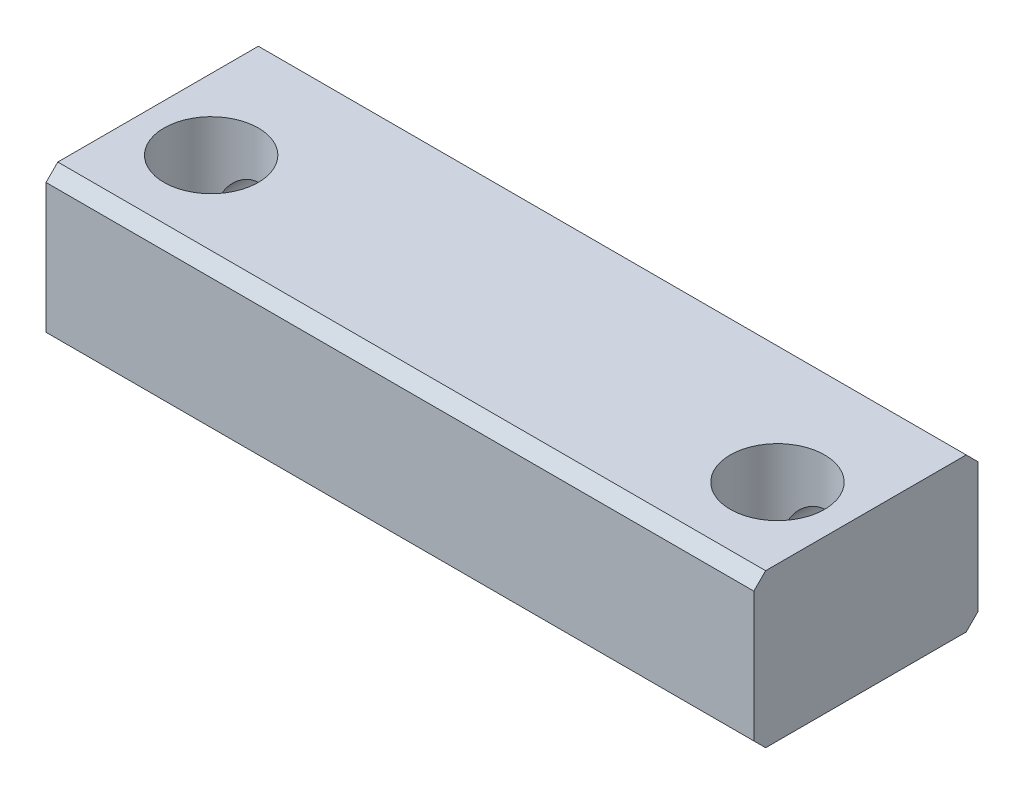
SolidWorks part; units mm, degrees
ref_plane "Front Plane" through (0, 0, 0) normal (0, 0, 1) x (1, 0, 0)
ref_plane "Top Plane" through (0, 0, 0) normal (0, 1, 0) x (1, 0, 0)
ref_plane "Right Plane" through (0, 0, 0) normal (1, 0, 0) x (0, 0, -1)
sketch "Sketch1" plane through (0, 0, 0) normal (0, 0, 1) x (1, 0, 0)
  line L1 (15, -3.25) -> (-15, -3.25)
  line L2 (15, -3.25) -> (15, 3.25)
  line L3 (15, 3.25) -> (-15, 3.25)
  line L4 (-15, -3.25) -> (-15, 3.25)
  line L5 (15, -3.25) -> (-15, 3.25) construction
  line L6 (15, 3.25) -> (-15, -3.25) construction
  point P0 (0, 0)
  dimension "D1" = 30
  dimension "D2" = 6.5
extrude "Boss-Extrude1" add sketch "Sketch1" along normal blind 9.5
sketch "Sketch2" plane through (0, 3.25, 0) normal (0, 1, 0) x (1, 0, 0)
  line L0 (15, 0) -> (-15, 0) construction
  line L1 (0, 0) -> (0, -9.5) construction
  line L2 (15, -9.5) -> (-15, -9.5) construction
  circle A0 centre (-12, -5.5) radius 2
  circle A1 centre (12, -5.5) radius 2
  dimension "D1" = 4
  dimension "D2" = 24
  dimension "D3" = 5.5
extrude "Cut-Extrude1" cut sketch "Sketch2" against normal through all
hole_wizard "M3 Tapped Hole1" positions "Sketch4" profile "Sketch3" tap size "M3" standard "GB"
sketch "Sketch4" plane through (0, 0, 0) normal (0, 0, -1) x (-1, 0, 0)
  line L0 (0, 3.25) -> (0, -3.25) construction
  line L1 (-15, 3.25) -> (15, 3.25) construction
  line L2 (15, -3.25) -> (-15, -3.25) construction
  line L4 (0, 0) -> (12, 0) construction
  point P0 (12, 0)
  point P1 (-12, 0)
  dimension "D1" = 24
cosmetic thread "Hole cosmetic thread1" parameters "D2"=3
cosmetic thread "Hole cosmetic thread2" parameters "D2"=3
sketch "Sketch3" plane through (-12, 0, 0) normal (1, 0, 0) x (0, 1, 0)
  line L0 (0, 0) -> (0, 3.5)
  line L1 (0, 3.5) -> (1.25, 3.5)
  line L2 (1.25, 3.5) -> (1.25, 0)
  line L5 (1.25, 0) -> (0, 0)
  line L11 (0, -6.35) -> (0, 107.95) construction
  dimension "通孔螺纹孔钻头直径" = 2.5
  dimension "通孔螺纹孔钻头深度" = 3.5
chamfer "Chamfer1" distance 0.5 angle 45 4 edges at (0, 3.25, 0) (0, 3.25, 9.5) (0, -3.25, 9.5) (0, -3.25, 0)
